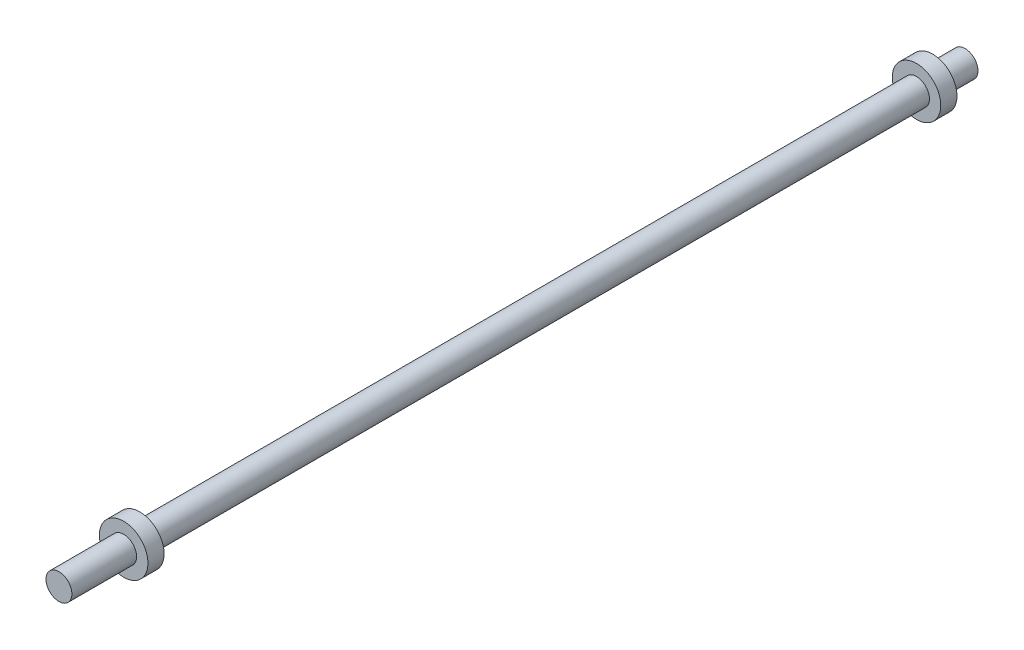
SolidWorks part; units mm, degrees
ref_plane "前视基准面" through (0, 0, 0) normal (0, 0, 1) x (1, 0, 0)
ref_plane "上视基准面" through (0, 0, 0) normal (0, 1, 0) x (1, 0, 0)
ref_plane "右视基准面" through (0, 0, 0) normal (1, 0, 0) x (0, 0, -1)
sketch "草图1" plane through (0, 0, 0) normal (0, 0, 1) x (1, 0, 0)
  circle A0 centre (0, 0) radius 4
  dimension "D1" = 8
extrude "凸台-拉伸1" add sketch "草图1" along normal mid plane 280
cosmetic thread "装饰螺纹线1" parameters "D1"=10, "D2"=6
sketch "草图2" plane through (0, 0, 140) normal (0, 0, 1) x (1, 0, 0)
  circle A0 centre (0, 0) radius 7.5
  dimension "D1" = 15
extrude "凸台-拉伸2" add sketch "草图2" against normal blind 5 from offset 20 offset against normal yes
sketch "草图3" plane through (0, 0, -140) normal (0, 0, -1) x (-1, 0, 0)
  circle A0 centre (0, 0) radius 7.5
  dimension "D1" = 15
extrude "凸台-拉伸3" add sketch "草图3" against normal blind 5 from offset 10
